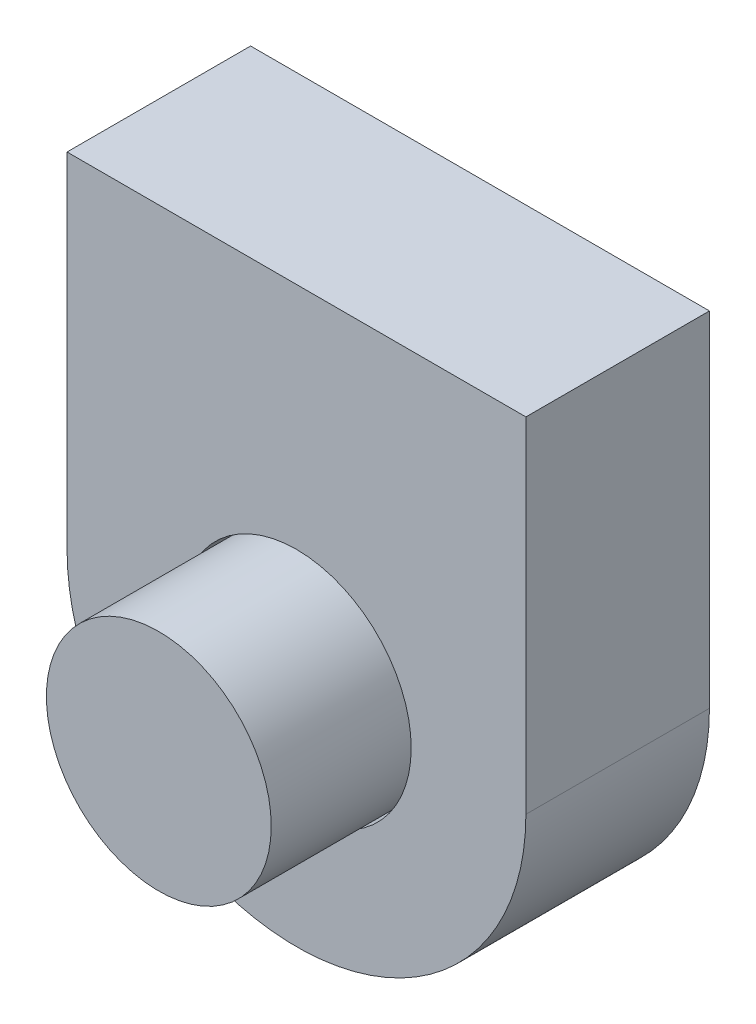
SolidWorks part; units mm, degrees
ref_plane "Front Plane" through (0, 0, 0) normal (0, 0, 1) x (1, 0, 0)
ref_plane "Top Plane" through (0, 0, 0) normal (0, 1, 0) x (1, 0, 0)
ref_plane "Right Plane" through (0, 0, 0) normal (1, 0, 0) x (0, 0, -1)
sketch "Sketch3" plane through (0, 0, 0) normal (0, 0, 1) x (1, 0, 0)
  line L0 (10, 0) -> (10, 15)
  line L1 (10, 15) -> (-10, 15)
  line L2 (-10, 15) -> (-10, 0)
  circle A0 centre (0, 0) radius 5
  arc A1 (-10, 0) -> (10, 0) centre (0, 0) ccw
extrude "Boss-Extrude1" add sketch "Sketch3" against normal blind 8 separate body
sketch "Sketch6" plane through (0, 0, 0) normal (0, 1, 0) x (1, 0, 0)
  line L0 (4.9, 8) -> (0, 8)
  line L1 (0, 8) -> (0, -6)
  line L2 (0, -6) -> (4.9, -6)
  line L3 (4.9, -6) -> (4.9, 8)
  line L4 (0, 8) -> (0, -6) construction
revolve "Revolve2" add sketch "Sketch6" angle 360 about L1
